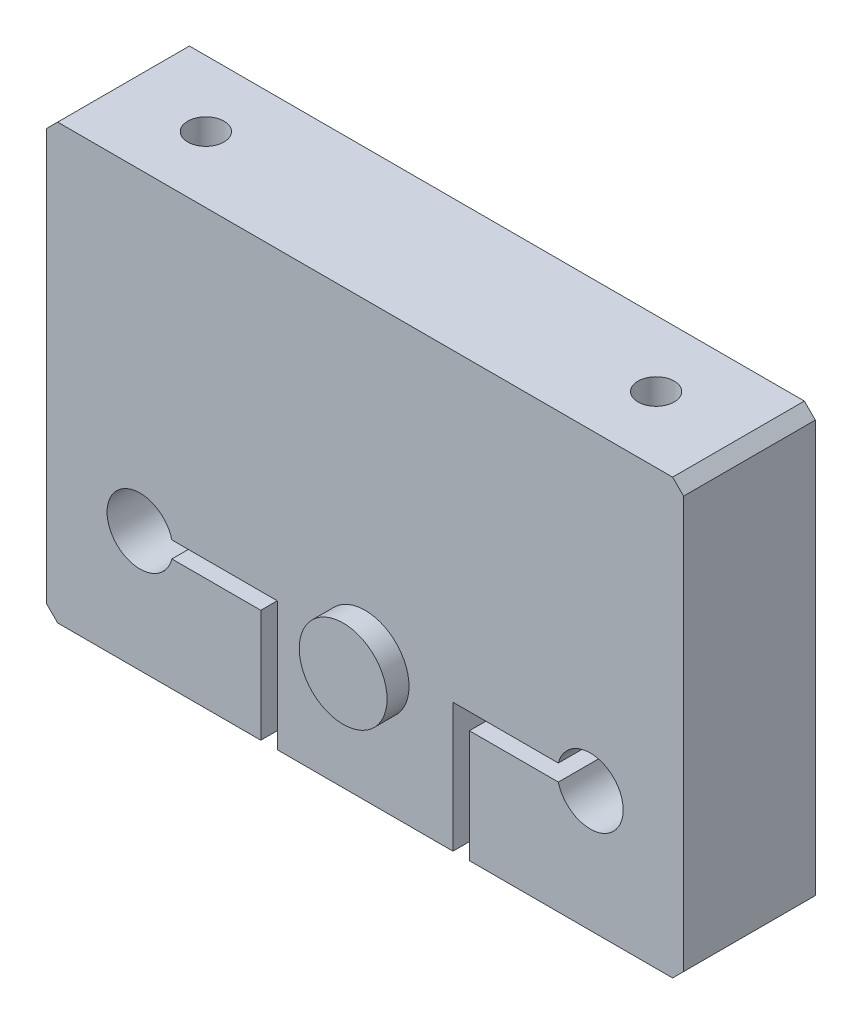
from build123d import *

# Parameters (mm, degrees)
BOSS_EXTRUDE1_DEPTH                     = 6
M4_TAPPED_HOLE1_AT_2_COUNT              = 2
M4_TAPPED_HOLE1_AT_2_PITCH              = 41
CBORE_FOR_M3_HEX_HEAD_BOLT1_D           = 3.5
CBORE_FOR_M3_HEX_HEAD_BOLT1_DEPTH       = 10.25
CBORE_FOR_M3_HEX_HEAD_BOLT1_CBORE_D     = 6
CBORE_FOR_M3_HEX_HEAD_BOLT1_CBORE_DEPTH = 3.5
M3_TAPPED_HOLE1_D                       = 2.5
M3_TAPPED_HOLE1_DEPTH                   = 7.5
M3_TAPPED_HOLE1_TIP                     = 0.751075774
M3_TAPPED_HOLE2_D                       = 2.5
M3_TAPPED_HOLE2_DEPTH                   = 8
M3_TAPPED_HOLE2_TIP                     = 0.751075774
SKETCH10_R                              = 4
CUT_EXTRUDE1_DEPTH                      = 3
SKETCH11_R                              = 4
BOSS_EXTRUDE2_DEPTH                     = 5
CHAMFER1_SIZE                           = 1


with BuildPart() as part:
    # Sketch1 → Boss-Extrude1 (new, symmetric)
    with BuildSketch(Plane.XY):
        with BuildLine():
            Line((-29, 19.75), (29, 19.75))
            Line((29, 19.75), (29, -19.75))
            Line((29, -19.75), (9.5, -19.75))
            Line((9.5, -19.75), (9.5, -9.5))
            Line((9.5, -9.5), (17.59526249, -9.5))
            ThreePointArc((17.59526249, -9.5), (23.5, -8.75), (17.59526249, -8))
            Line((17.59526249, -8), (8, -8))
            Line((8, -8), (8, -19.75))
            Line((8, -19.75), (-8, -19.75))
            Line((-8, -19.75), (-8, -8))
            Line((-8, -8), (-17.59526249, -8))
            ThreePointArc((-17.59526249, -8), (-23.5, -8.75), (-17.59526249, -9.5))
            Line((-17.59526249, -9.5), (-9.5, -9.5))
            Line((-9.5, -9.5), (-9.5, -19.75))
            Line((-9.5, -19.75), (-29, -19.75))
            Line((-29, -19.75), (-29, 19.75))
        make_face()
    extrude(amount=BOSS_EXTRUDE1_DEPTH, both=True)

    # Sketch2 → M4 Tapped Hole1 (revolve, cut)
    with BuildSketch(Plane(origin=(-20.5, 19.75, 0), x_dir=(0, 0, 1), z_dir=(1, 0, 0))):
        Polygon((0, 0), (0, 11.091420021), (1.65, 10.1), (1.65, 0), align=None)
    m4_tapped_hole1 = revolve(axis=Axis((-20.5, 26.1, 0), (0, -1, 0)), mode=Mode.SUBTRACT)

    # M4 Tapped Hole1 at 2: M4 Tapped Hole1 ×2
    with Locations(*[(i * M4_TAPPED_HOLE1_AT_2_PITCH, 0, 0) for i in range(1, M4_TAPPED_HOLE1_AT_2_COUNT)]):
        add(m4_tapped_hole1, mode=Mode.SUBTRACT)

    # Mirror1: M4 Tapped Hole1 across plane
    add(m4_tapped_hole1.mirror(Plane.ZX), mode=Mode.SUBTRACT)

    # Mirror1 copy 1 sketch → Mirror1 copy 1 (revolve, cut)
    with BuildSketch(Plane(origin=(20.5, -19.75, 0), x_dir=(0, 0, 1), z_dir=(1, 0, 0))):
        Polygon((0, 0), (0, -11.091420021), (1.65, -10.1), (1.65, 0), align=None)
    revolve(axis=Axis((20.5, -26.1, 0), (0, -1, 0)), mode=Mode.SUBTRACT)

    # CBORE for M3 Hex Head Bolt1
    with Locations(Plane.XZ.offset(19.75)):
        with Locations((-13.5, 0), (13.5, 0)):
            CounterBoreHole(CBORE_FOR_M3_HEX_HEAD_BOLT1_D / 2, CBORE_FOR_M3_HEX_HEAD_BOLT1_CBORE_D / 2, CBORE_FOR_M3_HEX_HEAD_BOLT1_CBORE_DEPTH, depth=CBORE_FOR_M3_HEX_HEAD_BOLT1_DEPTH)

    # M3 Tapped Hole1
    with Locations(Plane.XZ.offset(8)):
        with Locations((-13.5, 0), (13.5, 0)):
            Hole(M3_TAPPED_HOLE1_D / 2, depth=M3_TAPPED_HOLE1_DEPTH)
            with Locations((0, 0, -(M3_TAPPED_HOLE1_DEPTH + M3_TAPPED_HOLE1_TIP / 2))):  # 118° drill point
                Cone(0, M3_TAPPED_HOLE1_D / 2, M3_TAPPED_HOLE1_TIP, mode=Mode.SUBTRACT)

    # M3 Tapped Hole2
    with Locations(Plane.XZ.offset(19.75)):
        with Locations((25, 0)):
            Hole(M3_TAPPED_HOLE2_D / 2, depth=M3_TAPPED_HOLE2_DEPTH)
            with Locations((0, 0, -(M3_TAPPED_HOLE2_DEPTH + M3_TAPPED_HOLE2_TIP / 2))):  # 118° drill point
                Cone(0, M3_TAPPED_HOLE2_D / 2, M3_TAPPED_HOLE2_TIP, mode=Mode.SUBTRACT)

    # Sketch10 → Cut-Extrude1 (cut)
    with BuildSketch(Plane.XY.offset(6)):
        with Locations((0, -8.75)):
            Circle(SKETCH10_R)
    extrude(amount=-CUT_EXTRUDE1_DEPTH, mode=Mode.SUBTRACT)

    # Chamfer1
    chamfer1_edges = [part.edges().sort_by_distance(p)[0] for p in [
        (-29, -19.75, 0),
        (-29, 19.75, 0),
        (29, 19.75, 0),
        (29, -19.75, 0),
    ]]
    chamfer(chamfer1_edges, length=CHAMFER1_SIZE)


with BuildPart() as body_2:
    # Sketch11 → Boss-Extrude2 (new body)
    with BuildSketch(Plane.XY.offset(3)):
        with Locations((0, -8.75)):
            Circle(SKETCH11_R)
    extrude(amount=BOSS_EXTRUDE2_DEPTH)


solid = Compound([part.part, body_2.part])
